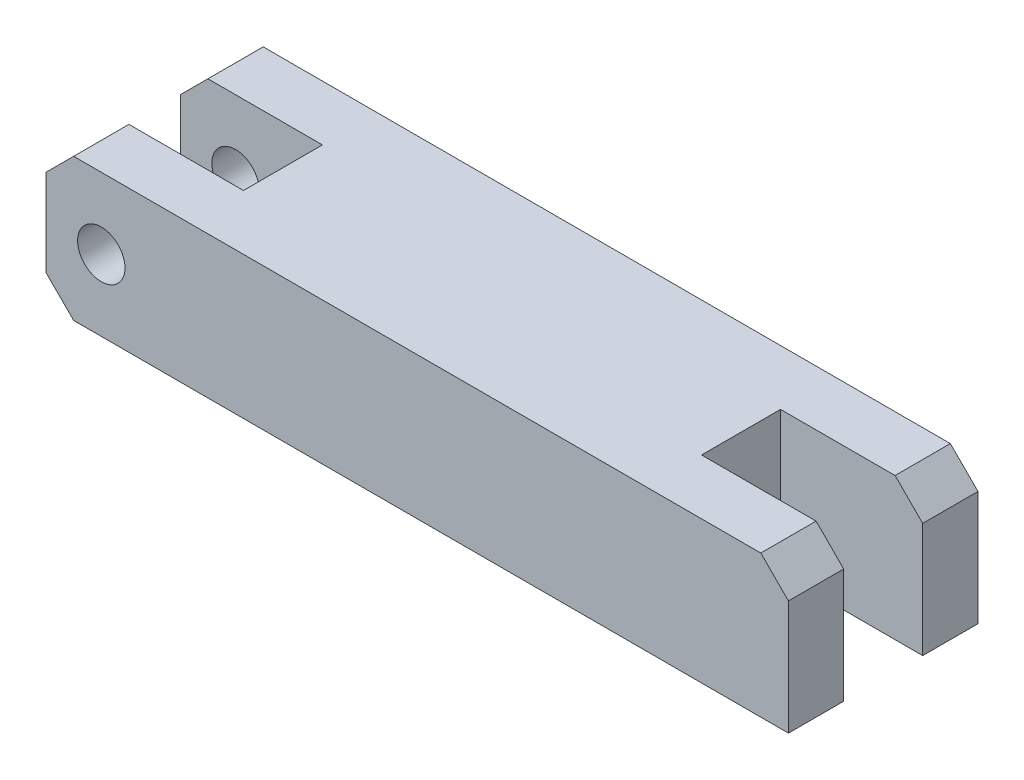
from build123d import *

# Parameters (mm, degrees)
SKETCH1_W           = 94
SKETCH1_H           = 24
BOSS_EXTRUDE1_DEPTH = 18
SKETCH2_W           = 36
SKETCH2_H           = 10
CUT_EXTRUDE1_DEPTH  = 70
CHAMFER1_SIZE       = 3.5
CHAMFER2_SIZE       = 3.5
SKETCH3_R           = 3
CUT_EXTRUDE2_DEPTH  = 70


with BuildPart() as part:
    # Sketch1 → Boss-Extrude1 (new body)
    with BuildSketch(Plane(origin=(0, 0, 0), x_dir=(1, 0, 0), z_dir=(0, 1, 0))):
        Rectangle(SKETCH1_W, SKETCH1_H)
    extrude(amount=BOSS_EXTRUDE1_DEPTH)

    # Sketch2 → Cut-Extrude1 (cut)
    with BuildSketch(Plane(origin=(0, 18, 0), x_dir=(1, 0, 0), z_dir=(0, 1, 0))):
        with Locations((-47, 0)):
            Rectangle(SKETCH2_W, SKETCH2_H)
        with Locations((47, 0)):
            Rectangle(SKETCH2_W, SKETCH2_H)
    extrude(amount=-CUT_EXTRUDE1_DEPTH, mode=Mode.SUBTRACT)

    # Chamfer1
    chamfer1_edges = [part.edges().sort_by_distance(p)[0] for p in [
        (47, 18, -8.5),
        (47, 18, 8.5),
    ]]
    chamfer(chamfer1_edges, length=CHAMFER1_SIZE)

    # Chamfer2
    chamfer2_edges = [part.edges().sort_by_distance(p)[0] for p in [
        (-47, 18, -8.5),
        (-47, 0, 8.5),
        (-47, 18, 8.5),
        (-47, 0, -8.5),
    ]]
    chamfer(chamfer2_edges, length=CHAMFER2_SIZE)

    # Sketch3 → Cut-Extrude2 (cut)
    with BuildSketch(Plane.XY.offset(12)):
        with Locations((-40, 9)):
            Circle(SKETCH3_R)
    extrude(amount=-CUT_EXTRUDE2_DEPTH, mode=Mode.SUBTRACT)


solid = part.part
